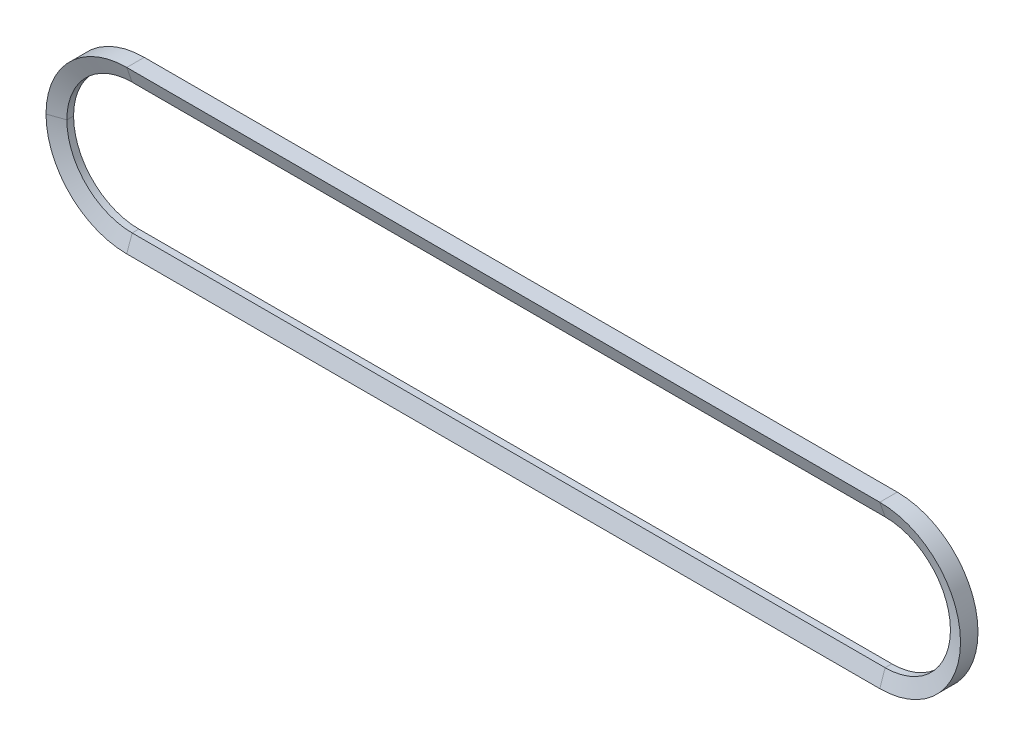
from build123d import *


with BuildPart() as part:
    # Sweep1: sweep along a path in Sketch1
    with BuildLine(Plane.XY) as sweep1_path:
        Line((-280, 48.55), (280, 48.55))
        ThreePointArc((280, 48.55), (328.55, 0), (280, -48.55))
        Line((280, -48.55), (-280, -48.55))
        ThreePointArc((-280, -48.55), (-328.55, 0), (-280, 48.55))
    # Sketch2 → Sweep1 (sweep)
    with BuildSketch(Plane(origin=(0, 0, 0), x_dir=(1, 0, 0), z_dir=(0, 1, 0))):
        Polygon((-328.55, 2.5), (-328.55, -2.5), (-340.05, -6.5), (-340.05, 6.5), align=None)
    sweep(path=sweep1_path.line)


solid = part.part
